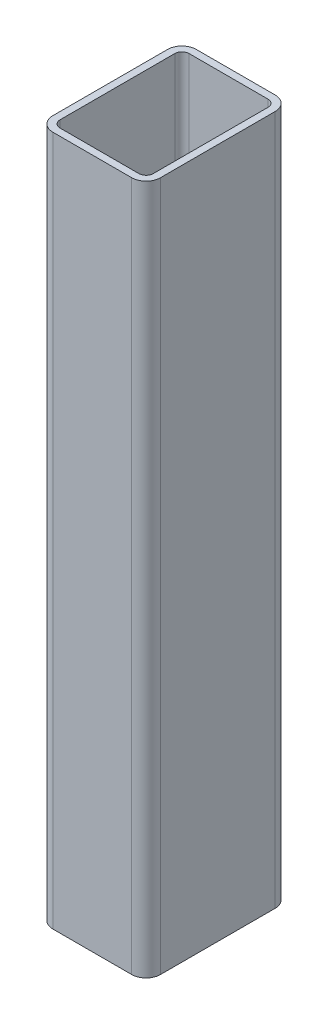
SolidWorks part; units mm, degrees
material "Q235B"
ref_plane "Front Plane" through (0, 0, 0) normal (0, 0, 1) x (1, 0, 0)
ref_plane "Top Plane" through (0, 0, 0) normal (0, 1, 0) x (1, 0, 0)
ref_plane "Right Plane" through (0, 0, 0) normal (1, 0, 0) x (0, 0, -1)
sketch "Sketch1" plane through (0, 0, 0) normal (0, 0, 1) x (1, 0, 0)
  line L0 (0, 0) -> (0, 385)
  dimension "D1" = 385
other "GB/T 6728-2002 rectangular hollow section 80X60X4(1)"
ref_plane "Plane1" through (0, 0, 0) normal (0, 1, 0) x (-1, 0, 0)
sketch "Sketch13" plane through (0, 0, 0) normal (0, 1, 0) x (-1, 0, 0)
  line L0 (-22, -36) -> (22, -36)
  line L1 (-26, -32) -> (-26, 32)
  line L2 (22, 36) -> (-22, 36)
  line L3 (26, 32) -> (26, -32)
  line L4 (-22, -40) -> (22, -40)
  line L5 (-30, -32) -> (-30, 32)
  line L6 (22, 40) -> (-22, 40)
  line L7 (30, 32) -> (30, -32)
  arc A0 (30, 32) -> (22, 40) centre (22, 32) ccw
  arc A1 (22, -40) -> (30, -32) centre (22, -32) ccw
  arc A2 (-30, -32) -> (-22, -40) centre (-22, -32) ccw
  arc A3 (-22, 40) -> (-30, 32) centre (-22, 32) ccw
  arc A4 (-22, 36) -> (-26, 32) centre (-22, 32) ccw
  arc A5 (26, 32) -> (22, 36) centre (22, 32) ccw
  arc A6 (22, -36) -> (26, -32) centre (22, -32) ccw
  arc A7 (-26, -32) -> (-22, -36) centre (-22, -32) ccw
  point P0 (0, 40)
  point P1 (30, 0)
  point P2 (0, -40)
  point P3 (-30, 0)
  point P4 (-30, 40)
  point P5 (30, 40)
  point P6 (30, -40)
  point P7 (-30, -40)
  point P8 (0, 0)
  point P33 (0, 0)
  dimension "D1" = 8
  dimension "Thickness" = 4
  dimension "V_leg" = 80
  dimension "H_leg" = 60
